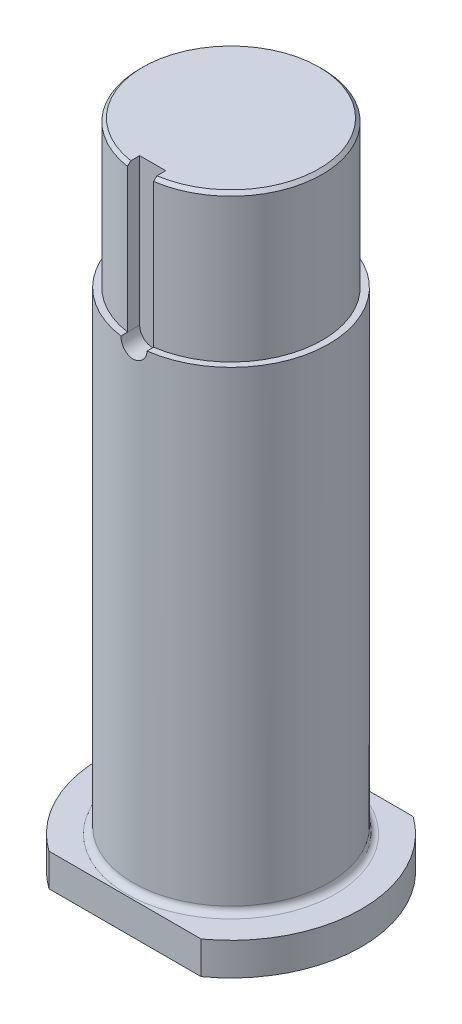
SolidWorks part; units mm, degrees
material "45#"
ref_plane "Front Plane" through (0, 0, 0) normal (0, 0, 1) x (1, 0, 0)
ref_plane "Top Plane" through (0, 0, 0) normal (0, 1, 0) x (1, 0, 0)
ref_plane "Right Plane" through (0, 0, 0) normal (1, 0, 0) x (0, 0, -1)
sketch "Sketch1" plane through (0, 0, 0) normal (0, 0, 1) x (1, 0, 0)
  line L0 (0, 0) -> (40, 0)
  line L1 (40, 0) -> (40, 10)
  line L2 (40, 10) -> (30, 10)
  line L3 (30, 10) -> (30, 155)
  line L4 (30, 155) -> (28, 155)
  line L5 (28, 155) -> (28, 200)
  line L6 (28, 200) -> (0, 200)
  line L7 (0, 200) -> (0, 0)
  line L8 (0, 0) -> (0, -14.4295) construction
  dimension "D1" = 80
  dimension "D2" = 60
  dimension "D3" = 56
  dimension "D4" = 45
  dimension "D5" = 200
  dimension "D6" = 10
revolve "Revolve1" add sketch "Sketch1" angle 360 about L8
cosmetic thread "Cosmetic Thread1" parameters "D1"=44, "D2"=50.046
sketch "Sketch2" plane through (0, 0, 0) normal (0, 1, 0) x (1, 0, 0)
  line L1 (65, -32.5) -> (-65, -32.5)
  line L2 (65, -32.5) -> (65, 32.5)
  line L3 (65, 32.5) -> (-65, 32.5)
  line L4 (-65, -32.5) -> (-65, 32.5)
  line L5 (65, -32.5) -> (-65, 32.5) construction
  line L6 (65, 32.5) -> (-65, -32.5) construction
  point P0 (0, 0)
  dimension "D1" = 65
  dimension "D2" = 130
extrude "Cut-Extrude1" cut sketch "Sketch2" along normal blind 10 flip side to cut
ref_plane "Plane1" through (0, 0, 24) normal (0, 0, 1) x (1, 0, 0)
sketch "Sketch3" plane through (0, 0, 24) normal (0, 0, 1) x (1, 0, 0)
  line L0 (0, 200) -> (0, 155) construction
  line L1 (28, 200) -> (-28, 200) construction
  line L2 (4, 200) -> (4, 155)
  line L3 (-4, 200) -> (-4, 155)
  line L4 (30, 155) -> (-30, 155) construction
  arc A0 (4, 200) -> (-4, 200) centre (0, 200) ccw
  arc A1 (-4, 155) -> (4, 155) centre (0, 155) ccw
  point P5 (0, 177.5)
  dimension "D1" = 8
extrude "Cut-Extrude2" cut sketch "Sketch3" along normal up to next
chamfer "Chamfer1" distance 1 angle 45 1 edges at (0, 200, -28)
fillet "Fillet1" [suppressed] radius 1
fillet "Fillet2" radius 2 1 edges at (0, 10, 30)
